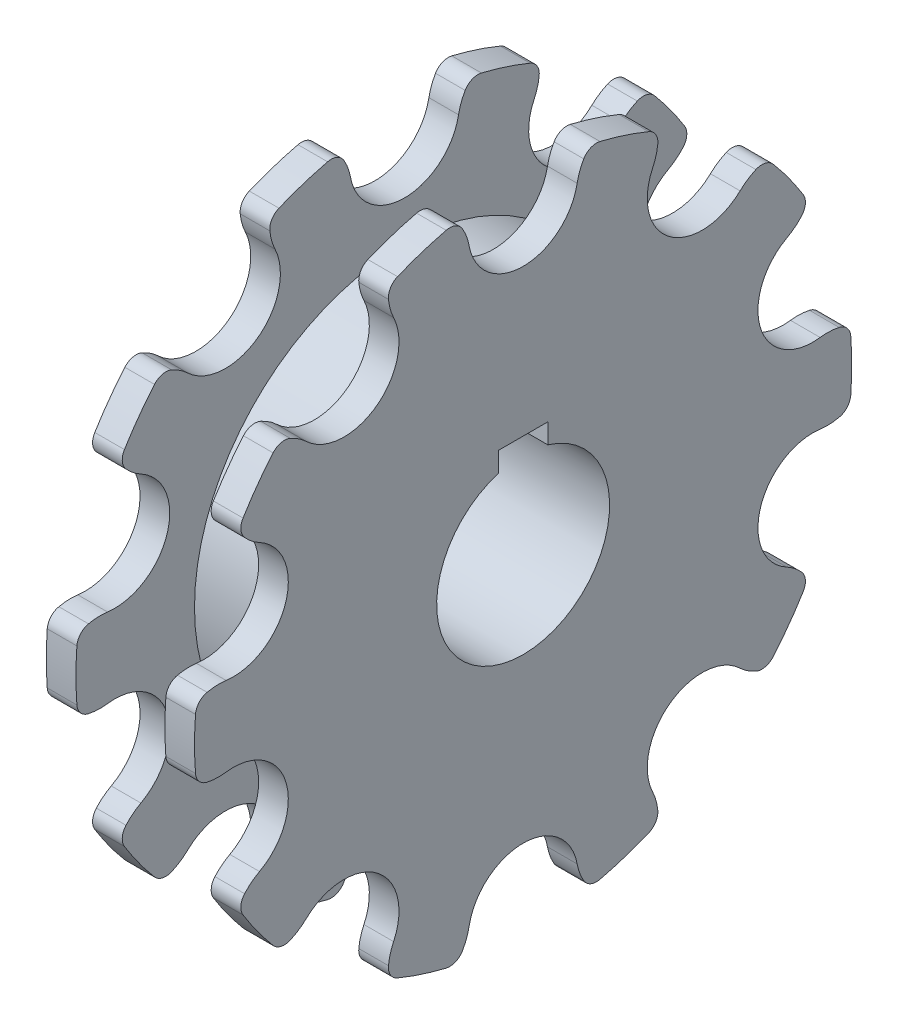
from build123d import *

# Parameters (mm, degrees)
SKETCH1_R                = 66.5
BOSS_EXTRUDE1_DEPTH      = 30
SKETCH2_R                = 17.5
CUT_EXTRUDE1_DEPTH       = 99.714234029
CUT_EXTRUDE2_DEPTH       = 99.714234029
CUT_EXTRUDE3_DEPTH       = 99.714234029
FILLET1_R                = 3
CIRPATTERN2_COUNT        = 10
FILLET1_OF_CIRPATTERN2_R = 3
SKETCH5_W                = 18
SKETCH5_H                = 30


with BuildPart() as part:
    # Sketch1 → Boss-Extrude1 (new body)
    with BuildSketch(Plane(origin=(0, 0, 0), x_dir=(0, 0, -1), z_dir=(1, 0, 0))):
        Circle(SKETCH1_R)
    extrude(amount=BOSS_EXTRUDE1_DEPTH)

    # Sketch2 → Cut-Extrude1 (cut, through all)
    with BuildSketch(Plane(origin=(30, 0, 0), x_dir=(0, 0, -1), z_dir=(1, 0, 0))):
        Circle(SKETCH2_R)
    extrude(amount=-CUT_EXTRUDE1_DEPTH, mode=Mode.SUBTRACT)

    # Sketch3 → Cut-Extrude2 (cut, through all)
    with BuildSketch(Plane(origin=(30, 0, 0), x_dir=(0, 0, -1), z_dir=(1, 0, 0))):
        with BuildLine():
            Line((-5, 16.770509831), (-5, 20.8))
            Line((-5, 20.8), (5, 20.8))
            Line((5, 20.8), (5, 16.770509831))
            ThreePointArc((5, 16.770509831), (0, 17.5), (-5, 16.770509831))
        make_face()
    extrude(amount=-CUT_EXTRUDE2_DEPTH, mode=Mode.SUBTRACT)

    # Sketch4 → Cut-Extrude3 (cut, through all)
    with BuildSketch(Plane(origin=(30, 0, 0), x_dir=(0, 0, -1), z_dir=(1, 0, 0))):
        with BuildLine():
            ThreePointArc((-10.932860029, 59.646054745), (0, 50.535), (10.932860029, 59.646054745))
            ThreePointArc((10.932860029, 59.646054745), (11.895576941, 62.555303076), (13.616126786, 65.091098403))
            ThreePointArc((13.616126786, 65.091098403), (0, 66.5), (-13.616126786, 65.091098403))
            ThreePointArc((-13.616126786, 65.091098403), (-11.895576941, 62.555303076), (-10.932860029, 59.646054745))
        make_face()
    cut_extrude3 = extrude(amount=-CUT_EXTRUDE3_DEPTH, mode=Mode.SUBTRACT)

    # Fillet1
    fillet1_edges = [part.edges().sort_by_distance(p)[0] for p in [
        (15, 65.091098403, 13.616126786),
        (15, 65.091098403, -13.616126786),
    ]]
    fillet(fillet1_edges, radius=FILLET1_R)

    # CirPattern2: Cut-Extrude3 ×10 about axis
    cirpattern2_axis = Axis((0, 0, 0), (1, 0, 0))
    for i in range(1, CIRPATTERN2_COUNT):
        add(cut_extrude3.rotate(cirpattern2_axis, i * 360 / CIRPATTERN2_COUNT), mode=Mode.SUBTRACT)

    # Fillet1 of CirPattern2
    fillet1_of_cirpattern2_edges = [part.edges().sort_by_distance(p)[0] for p in [
        (15, 44.656446273, 49.275265664),
        (15, 60.663163309, 27.24390973),
        (15, 7.164549483, 66.112927864),
        (15, 33.063961696, 57.697698715),
        (15, -33.063961696, 57.697698715),
        (15, -7.164549483, 66.112927864),
        (15, -60.663163309, 27.24390973),
        (15, -44.656446273, 49.275265664),
        (15, -65.091098403, -13.616126786),
        (15, -65.091098403, 13.616126786),
        (15, -44.656446273, -49.275265664),
        (15, -60.663163309, -27.24390973),
        (15, -7.164549483, -66.112927864),
        (15, -33.063961696, -57.697698715),
        (15, 33.063961696, -57.697698715),
        (15, 7.164549483, -66.112927864),
        (15, 60.663163309, -27.24390973),
        (15, 44.656446273, -49.275265664),
    ]]
    fillet(fillet1_of_cirpattern2_edges, radius=FILLET1_OF_CIRPATTERN2_R)

    # Sketch5 → Cut-Revolve1 (revolve, cut)
    with BuildSketch(Plane(origin=(0, 0, 0), x_dir=(1, 0, 0), z_dir=(0, 1, 0)), mode=Mode.PRIVATE) as cut_revolve1_sk:
        with Locations((15, 57.5)):
            Rectangle(SKETCH5_W, SKETCH5_H)
    revolve(cut_revolve1_sk.sketch.rotate(Axis((0, 0, 0), (1, 0, 0)), 180), axis=Axis((0, 0, 0), (1, 0, 0)), mode=Mode.SUBTRACT)


solid = part.part
